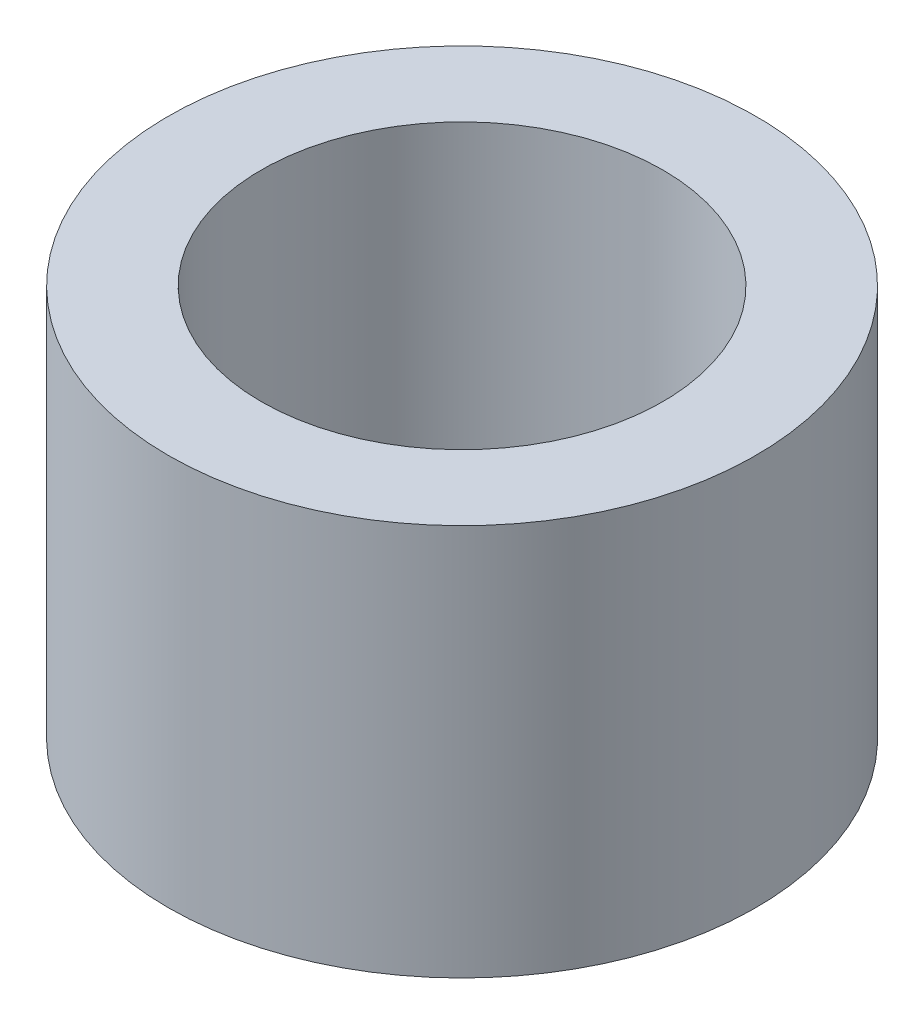
SolidWorks part; units mm, degrees
material "普通碳钢"
ref_plane "前视" through (0, 0, 0) normal (0, 0, 1) x (1, 0, 0)
ref_plane "上视" through (0, 0, 0) normal (0, 1, 0) x (1, 0, 0)
ref_plane "右视" through (0, 0, 0) normal (1, 0, 0) x (0, 0, -1)
sketch "草图1" plane through (0, 0, 0) normal (0, 1, 0) x (1, 0, 0)
  circle A0 centre (0, 0) radius 10.25
  circle A1 centre (0, 0) radius 15
  dimension "D1" = 20.5
  dimension "D2" = 30
extrude "凸台-拉伸1" add sketch "草图1" along normal blind 20
